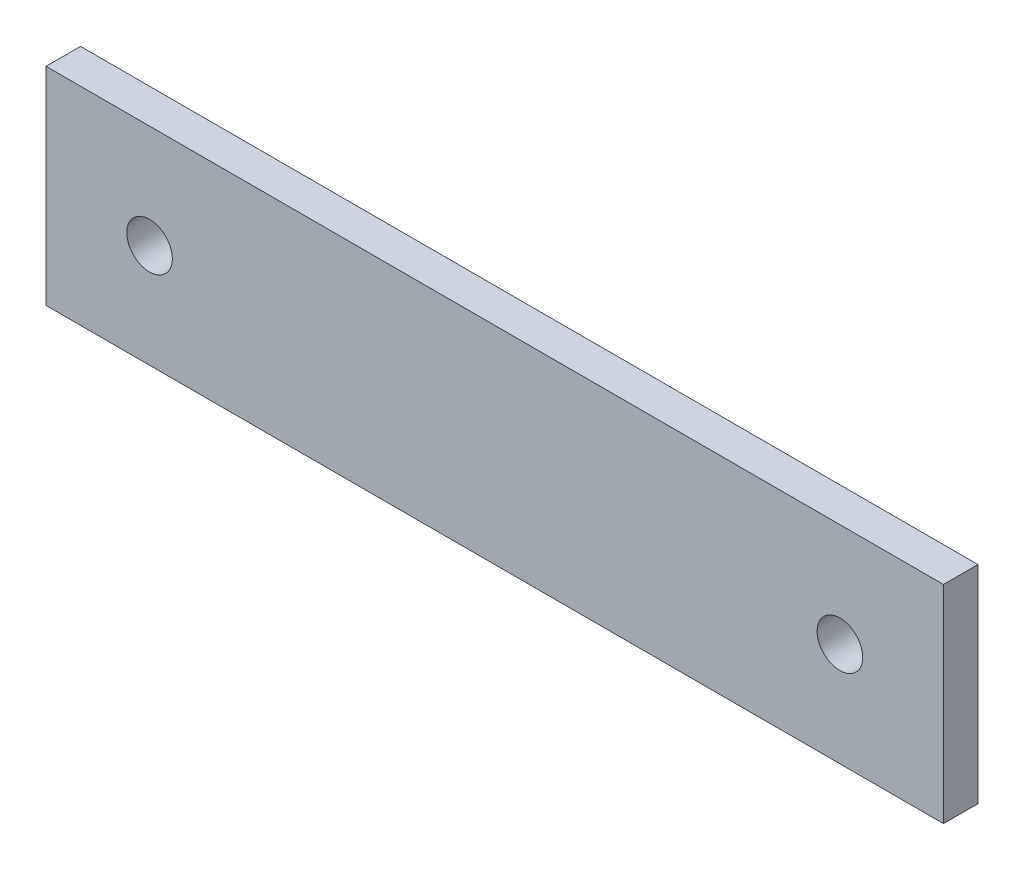
from build123d import *

# Parameters (mm, degrees)
SKETCH_1_W      = 130
SKETCH_1_H      = 30
SKETCH_1_R      = 3.3
EXTRUDE_1_DEPTH = 5


with BuildPart() as part:
    # 草图1 → 凸台-拉伸1 (new body)
    with BuildSketch(Plane.XY):
        Rectangle(SKETCH_1_W, SKETCH_1_H)
        with Locations((-50, 0)):
            Circle(SKETCH_1_R, mode=Mode.SUBTRACT)
        with Locations((50, 0)):
            Circle(SKETCH_1_R, mode=Mode.SUBTRACT)
    extrude(amount=EXTRUDE_1_DEPTH)


solid = part.part
